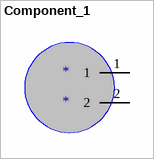
[diagram p0: symbol Component_1]
# Altium schematic symbol library MISC86340-21.SchLib: 1 symbol
Pins are listed as number, name and electrical type; pins without a type are passive.


## Component_1
designator *
footprint mimi
pins: 1, 2